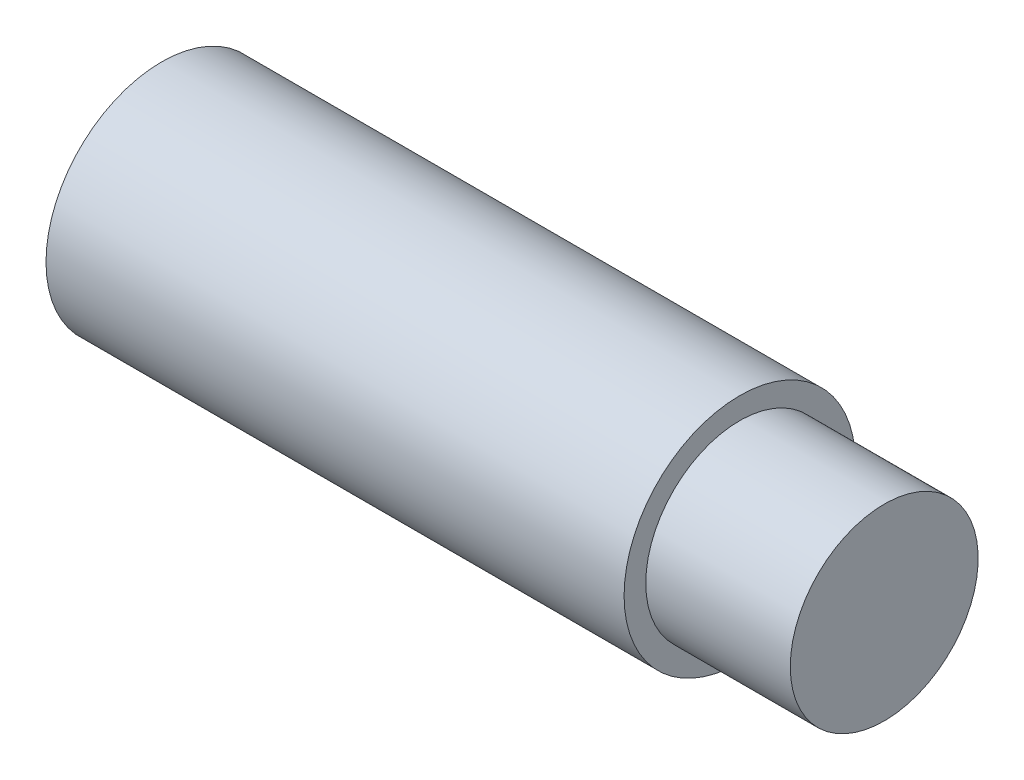
SolidWorks part; units mm, degrees
ref_plane "Front Plane" through (0, 0, 0) normal (0, 0, 1) x (1, 0, 0)
ref_plane "Top Plane" through (0, 0, 0) normal (0, 1, 0) x (1, 0, 0)
ref_plane "Right Plane" through (0, 0, 0) normal (1, 0, 0) x (0, 0, -1)
sketch "Sketch1" plane through (0, 0, 0) normal (0, 0, 1) x (1, 0, 0)
  line L0 (0, 0) -> (50, 0) construction
  line L1 (0, 0) -> (0, 8)
  line L2 (0, 8) -> (40, 8)
  line L3 (40, 8) -> (40, 6.5)
  line L4 (40, 6.5) -> (50, 6.5)
  line L5 (50, 6.5) -> (50, 0)
  line L6 (0, 0) -> (50, 0)
  dimension "D1" = 10
  dimension "D2" = 8
  dimension "D3" = 6.5
  dimension "D4" = 50
revolve "Revolve1" add sketch "Sketch1" angle 360 about L0
